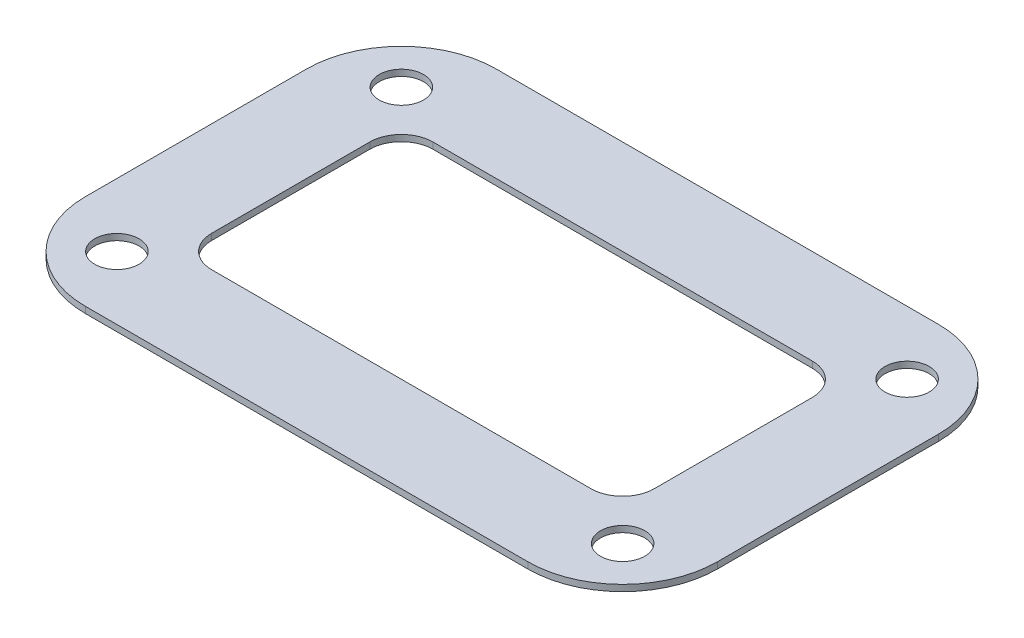
SolidWorks part; units mm, degrees
ref_plane "Front Plane" through (0, 0, 0) normal (0, 0, 1) x (1, 0, 0)
ref_plane "Top Plane" through (0, 0, 0) normal (0, 1, 0) x (1, 0, 0)
ref_plane "Right Plane" through (0, 0, 0) normal (1, 0, 0) x (0, 0, -1)
sketch "Sketch1" plane through (0, 0, 0) normal (0, 1, 0) x (1, 0, 0)
  line L1 (-35, 32.5) -> (35, 32.5)
  line L2 (-50, 17.5) -> (-50, -17.5)
  line L3 (-35, -32.5) -> (35, -32.5)
  line L4 (50, 17.5) -> (50, -17.5)
  line L5 (-50, 32.5) -> (50, -32.5) construction
  line L6 (-50, -32.5) -> (50, 32.5) construction
  arc A0 (35, 32.5) -> (50, 17.5) centre (35, 17.5) cw
  arc A1 (-50, -17.5) -> (-35, -32.5) centre (-35, -17.5) ccw
  arc A2 (-35, 32.5) -> (-50, 17.5) centre (-35, 17.5) ccw
  arc A3 (35, -32.5) -> (50, -17.5) centre (35, -17.5) ccw
  point P0 (0, 0)
  dimension "D3" = 15
  dimension "D1" = 65
  dimension "D2" = 100
extrude "Boss-Extrude1" add sketch "Sketch1" along normal blind 1
sketch "Sketch2" plane through (0, 1, 0) normal (0, 1, 0) x (1, 0, 0)
  line L1 (-30, 17.5) -> (30, 17.5)
  line L2 (-35, 12.5) -> (-35, -12.5)
  line L3 (-30, -17.5) -> (30, -17.5)
  line L4 (35, 12.5) -> (35, -12.5)
  line L5 (-35, 17.5) -> (35, -17.5) construction
  line L6 (-35, -17.5) -> (35, 17.5) construction
  arc A0 (30, 17.5) -> (35, 12.5) centre (30, 12.5) cw
  arc A1 (-35, -12.5) -> (-30, -17.5) centre (-30, -12.5) ccw
  arc A2 (-30, 17.5) -> (-35, 12.5) centre (-30, 12.5) ccw
  arc A3 (30, -17.5) -> (35, -12.5) centre (30, -12.5) ccw
  point P0 (0, 0)
  dimension "D3" = 5
  dimension "D1" = 35
  dimension "D2" = 70
extrude "Cut-Extrude1" cut sketch "Sketch2" against normal through all
hole_wizard "Hole1" positions "3DSketch1" profile "Sketch3" legacy end condition up to next
sketch3d "3DSketch1"
  point P0 (-40, 1, -22.5)
  dimension "D1" = 22.5
  dimension "D2" = 40
sketch "Sketch3" plane through (-40, 1, -22.5) normal (1, 0, 0) x (0, 0, 1)
  line L0 (0, 0) -> (0, 1.001)
  line L1 (0, 1.001) -> (3.5, 1.001)
  line L2 (3.5, 1.001) -> (3.5, 0)
  line L3 (3.5, 0) -> (0, 0)
  line L4 (0, 110) -> (0, -10) construction
  dimension "直径" = 7
  dimension "深度" = 1.001
pattern_linear "LPattern1" count 2 spacing 80 along (1, 0, 0) count 2 spacing 45 along (0, 0, 1) of "Hole1"
